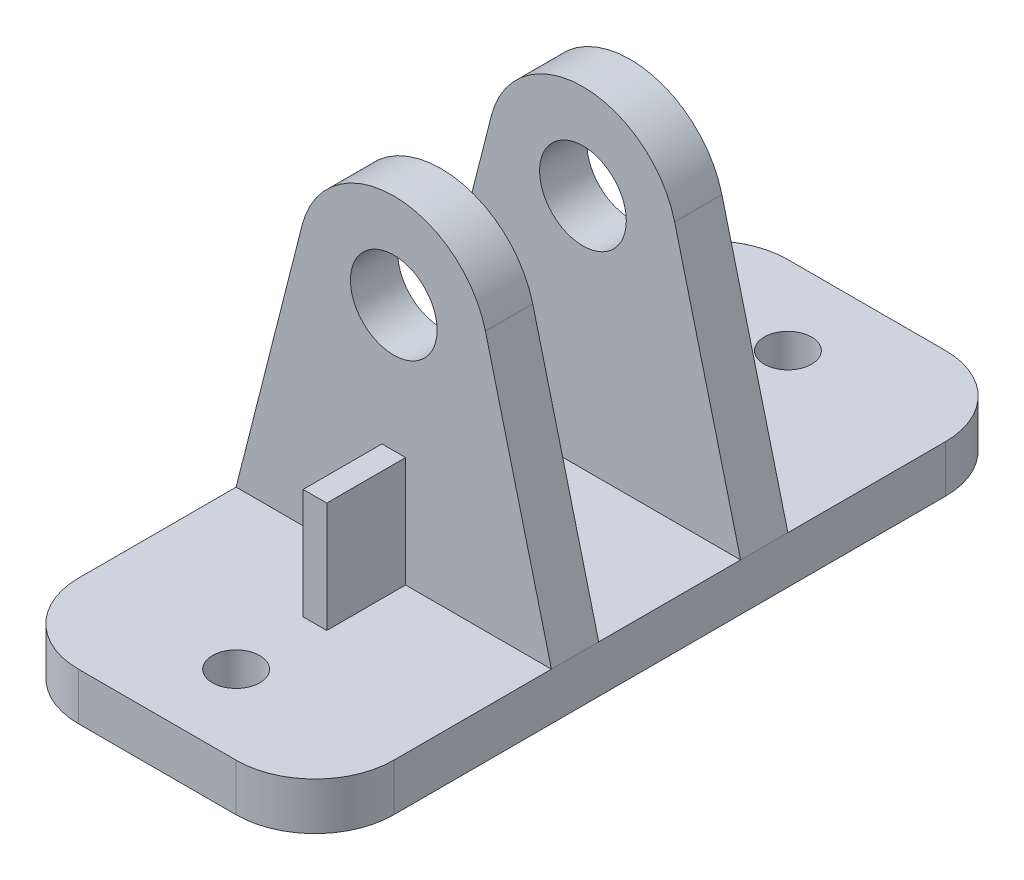
from build123d import *

# Parameters (mm, degrees)
SKETCH_1_W           = 200
SKETCH_1_H           = 150
BOSS_EXTRUDE_1_DEPTH = 30
SKETCH_2_R           = 27.5
BOSS_EXTRUDE_2_DEPTH = 30
SKETCH_4_W           = 15
SKETCH_4_H           = 100
BOSS_EXTRUDE_3_DEPTH = 50
SKETCH_5_W           = 200
SKETCH_5_H           = 450
SKETCH_5_R           = 15
BOSS_EXTRUDE_4_DEPTH = 30
FILLET_1_R           = 50


with BuildPart() as part:
    # Sketch 1 → Boss-Extrude 1 (new body)
    with BuildSketch(Plane(origin=(0, 0, 0), x_dir=(1, 0, 0), z_dir=(0, 1, 0))):
        Rectangle(SKETCH_1_W, SKETCH_1_H)
    extrude(amount=BOSS_EXTRUDE_1_DEPTH)

    # Sketch 2 → Boss-Extrude 2 (add)
    with BuildSketch(Plane.XY.offset(75)):
        with BuildLine():
            Line((-58.153846154, 194.769230769), (-100, 30))
            Line((-100, 30), (100, 30))
            Line((100, 30), (58.153846154, 194.769230769))
            ThreePointArc((58.153846154, 194.769230769), (0, 240), (-58.153846154, 194.769230769))
        make_face()
        with Locations((0, 180)):
            Circle(SKETCH_2_R, mode=Mode.SUBTRACT)
    boss_extrude_2 = extrude(amount=-BOSS_EXTRUDE_2_DEPTH)

    # Sketch 4 → Boss-Extrude 3 (add)
    with BuildSketch(Plane.XY.offset(75)):
        with Locations((0, 50)):
            Rectangle(SKETCH_4_W, SKETCH_4_H)
    boss_extrude_3 = extrude(amount=BOSS_EXTRUDE_3_DEPTH)

    # Mirror 1: Boss-Extrude 2, Boss-Extrude 3 across plane
    add(boss_extrude_2.mirror(Plane.XY))
    add(boss_extrude_3.mirror(Plane.XY))

    # Sketch 5 → Boss-Extrude 4 (add)
    with BuildSketch(Plane.XZ):
        Rectangle(SKETCH_5_W, SKETCH_5_H)
        with Locations(Location((0, -175, 0), (0, 0, 270))):
            Circle(SKETCH_5_R, mode=Mode.SUBTRACT)
        with Locations(Location((0, 175, 0), (0, 0, 270))):
            Circle(SKETCH_5_R, mode=Mode.SUBTRACT)
    extrude(amount=-BOSS_EXTRUDE_4_DEPTH)

    # Fillet 1
    fillet_1_edges = [part.edges().sort_by_distance(p)[0] for p in [
        (-100, 15, -225),
        (100, 15, 225),
        (100, 15, -225),
        (-100, 15, 225),
    ]]
    fillet(fillet_1_edges, radius=FILLET_1_R)


solid = part.part
